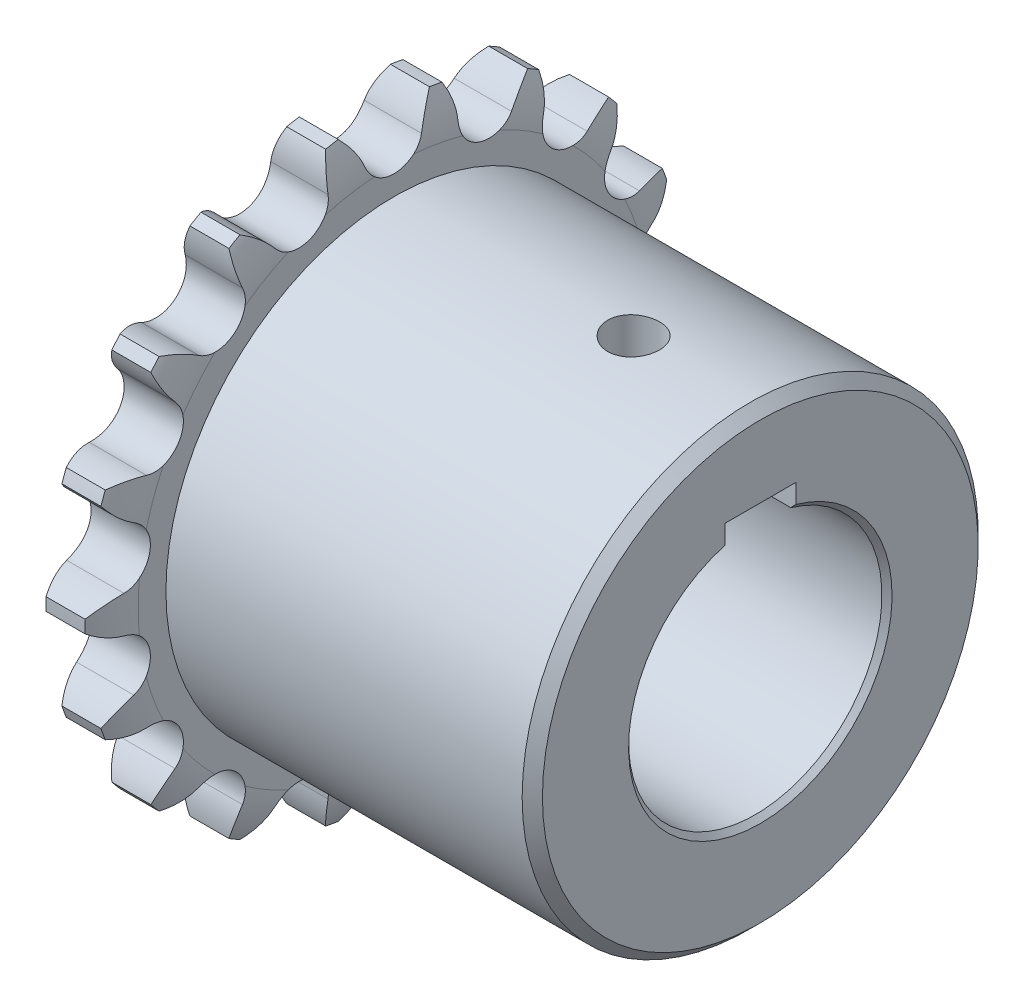
from build123d import *

# Parameters (mm, degrees)
EXTRUDE2_DEPTH         = 119.367739693
M12_TAPPED_HOLE1_D     = 10.2
M12_TAPPED_HOLE1_DEPTH = 42.75
M12_TAPPED_HOLE1_TIP   = 3.064389157
CUT_EXTRUDE1_DEPTH     = 33
CIRPATTERN1_COUNT      = 18
CHAMFER1_SIZE          = 1


with BuildPart() as part:
    # Sketch1 → Revolve1 (revolve)
    with BuildSketch(Plane.XY, mode=Mode.PRIVATE) as revolve1_sk:
        with BuildLine():
            Line((84, -43), (82, -45))
            Line((82, -45), (11.7, -45))
            Line((11.7, -45), (11.7, -50.484718626))
            ThreePointArc((11.7, -50.484718626), (11.193242009, -54.843617569), (9.7, -58.97))
            Line((9.7, -58.97), (2, -58.97))
            ThreePointArc((2, -58.97), (0.506757991, -54.843617569), (0, -50.484718626))
            Line((0, -50.484718626), (0, -25))
            Line((0, -25), (84, -25))
            Line((84, -25), (84, -43))
        make_face()
    revolve(revolve1_sk.sketch.rotate(Axis((0, 0, 0), (1, 0, 0)), 270), axis=Axis((0, 0, 0), (1, 0, 0)))

    # Sketch4 → Extrude2 (cut, through all)
    with BuildSketch(Plane(origin=(84, 0, 0), x_dir=(0, 0, -1), z_dir=(1, 0, 0))):
        with BuildLine():
            Line((-7, 28.8), (-7, 24))
            ThreePointArc((-7, 24), (0, 25), (7, 24))
            Line((7, 24), (7, 28.8))
            Line((7, 28.8), (-7, 28.8))
        make_face()
    extrude(amount=-EXTRUDE2_DEPTH, mode=Mode.SUBTRACT)

    # M12 Tapped Hole1
    with Locations(Plane.XZ.offset(-28.8)):
        with Locations((59, 0)):
            Hole(M12_TAPPED_HOLE1_D / 2, depth=M12_TAPPED_HOLE1_DEPTH)
            with Locations((0, 0, -(M12_TAPPED_HOLE1_DEPTH + M12_TAPPED_HOLE1_TIP / 2))):  # 118° drill point
                Cone(0, M12_TAPPED_HOLE1_D / 2, M12_TAPPED_HOLE1_TIP, mode=Mode.SUBTRACT)

    # Sketch7 → Cut-Extrude1 (cut)
    with BuildSketch(Plane.ZY):
        with BuildLine():
            ThreePointArc((-5.628968769, 52.911617485), (0, 48.9), (5.628968769, 52.911617485))
            ThreePointArc((5.628968769, 52.911617485), (7.006728654, 55.788673273), (9, 58.279163515))
            ThreePointArc((9, 58.279163515), (0, 58.97), (-9, 58.279163515))
            ThreePointArc((-9, 58.279163515), (-7.006728654, 55.788673273), (-5.628968769, 52.911617485))
        make_face()
    cut_extrude1 = extrude(amount=-CUT_EXTRUDE1_DEPTH, mode=Mode.SUBTRACT)

    # CirPattern1: Cut-Extrude1 ×18 about axis
    cirpattern1_axis = Axis((0, 0, 0), (1, 0, 0))
    for i in range(1, CIRPATTERN1_COUNT):
        add(cut_extrude1.rotate(cirpattern1_axis, i * 360 / CIRPATTERN1_COUNT), mode=Mode.SUBTRACT)

    # Chamfer1
    chamfer1_edges = [part.edges().sort_by_distance(p)[0] for p in [
        (0, -25, 0),
        (84, -25, 0),
    ]]
    chamfer(chamfer1_edges, length=CHAMFER1_SIZE)


solid = part.part
